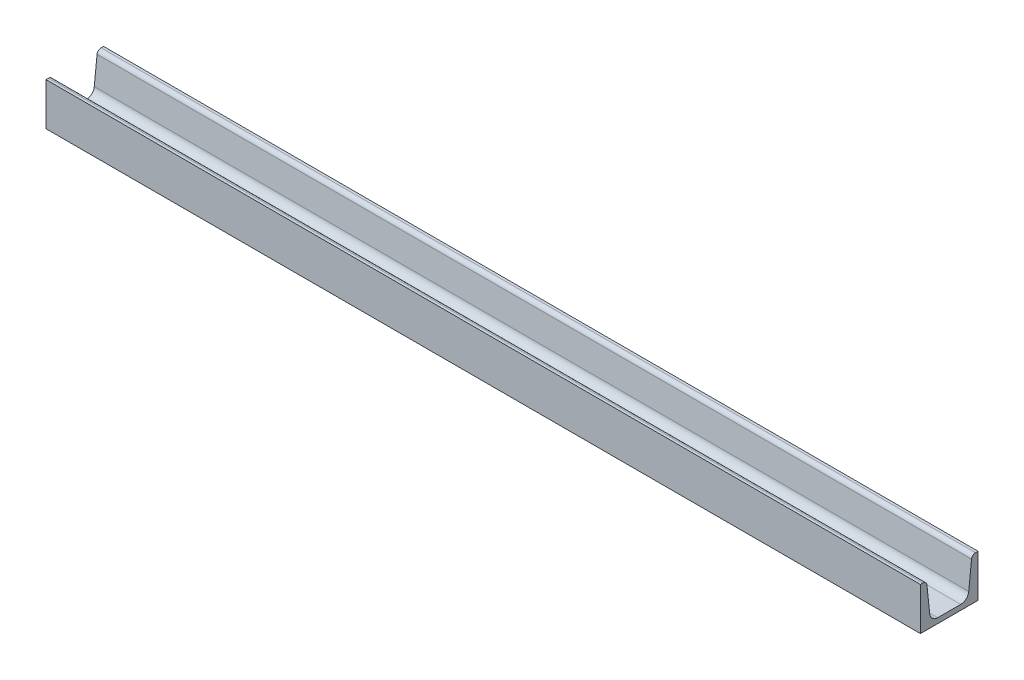
from build123d import *

# Parameters (mm, degrees)
GB_T_707_1988_HOT_ROLLED_CHANNEL_05_1_DEPTH = 760


with BuildPart() as part:
    # Sketch1 → GB/T 707-1988 hot-rolled channel 05(1) (new body)
    with BuildSketch(Plane.YZ.offset(-380)):
        with BuildLine():
            Line((37, 50), (0, 50))
            Line((0, 50), (0, 0))
            Line((0, 0), (37, 0))
            Line((37, 0), (37, 2.140642022))
            ThreePointArc((37, 2.140642022), (36.101006889, 4.482599144), (33.865849621, 5.621468656))
            Line((33.865849621, 5.621468656), (10.768300757, 8.049118866))
            ThreePointArc((10.768300757, 8.049118866), (6.297986222, 10.326857889), (4.5, 15.010772133))
            Line((4.5, 15.010772133), (4.5, 34.989227867))
            ThreePointArc((4.5, 34.989227867), (6.297986222, 39.673142111), (10.768300757, 41.950881134))
            Line((10.768300757, 41.950881134), (33.865849621, 44.378531344))
            ThreePointArc((33.865849621, 44.378531344), (36.101006889, 45.517400856), (37, 47.859357978))
            Line((37, 47.859357978), (37, 50))
        make_face()
    extrude(amount=GB_T_707_1988_HOT_ROLLED_CHANNEL_05_1_DEPTH)


solid = part.part
